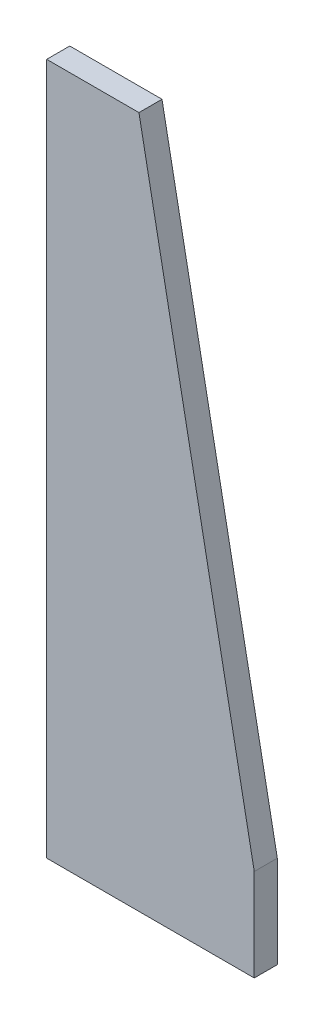
from build123d import *

# Parameters (mm, degrees)
EXTRUDE_1_DEPTH = 2.5


with BuildPart() as part:
    # 草图1 → 凸台-拉伸1 (new, symmetric)
    with BuildSketch(Plane.XY):
        Polygon((0, 0), (0, 150), (20, 150), (45, 20), (45, 0), align=None)
    extrude(amount=EXTRUDE_1_DEPTH, both=True)


solid = part.part
